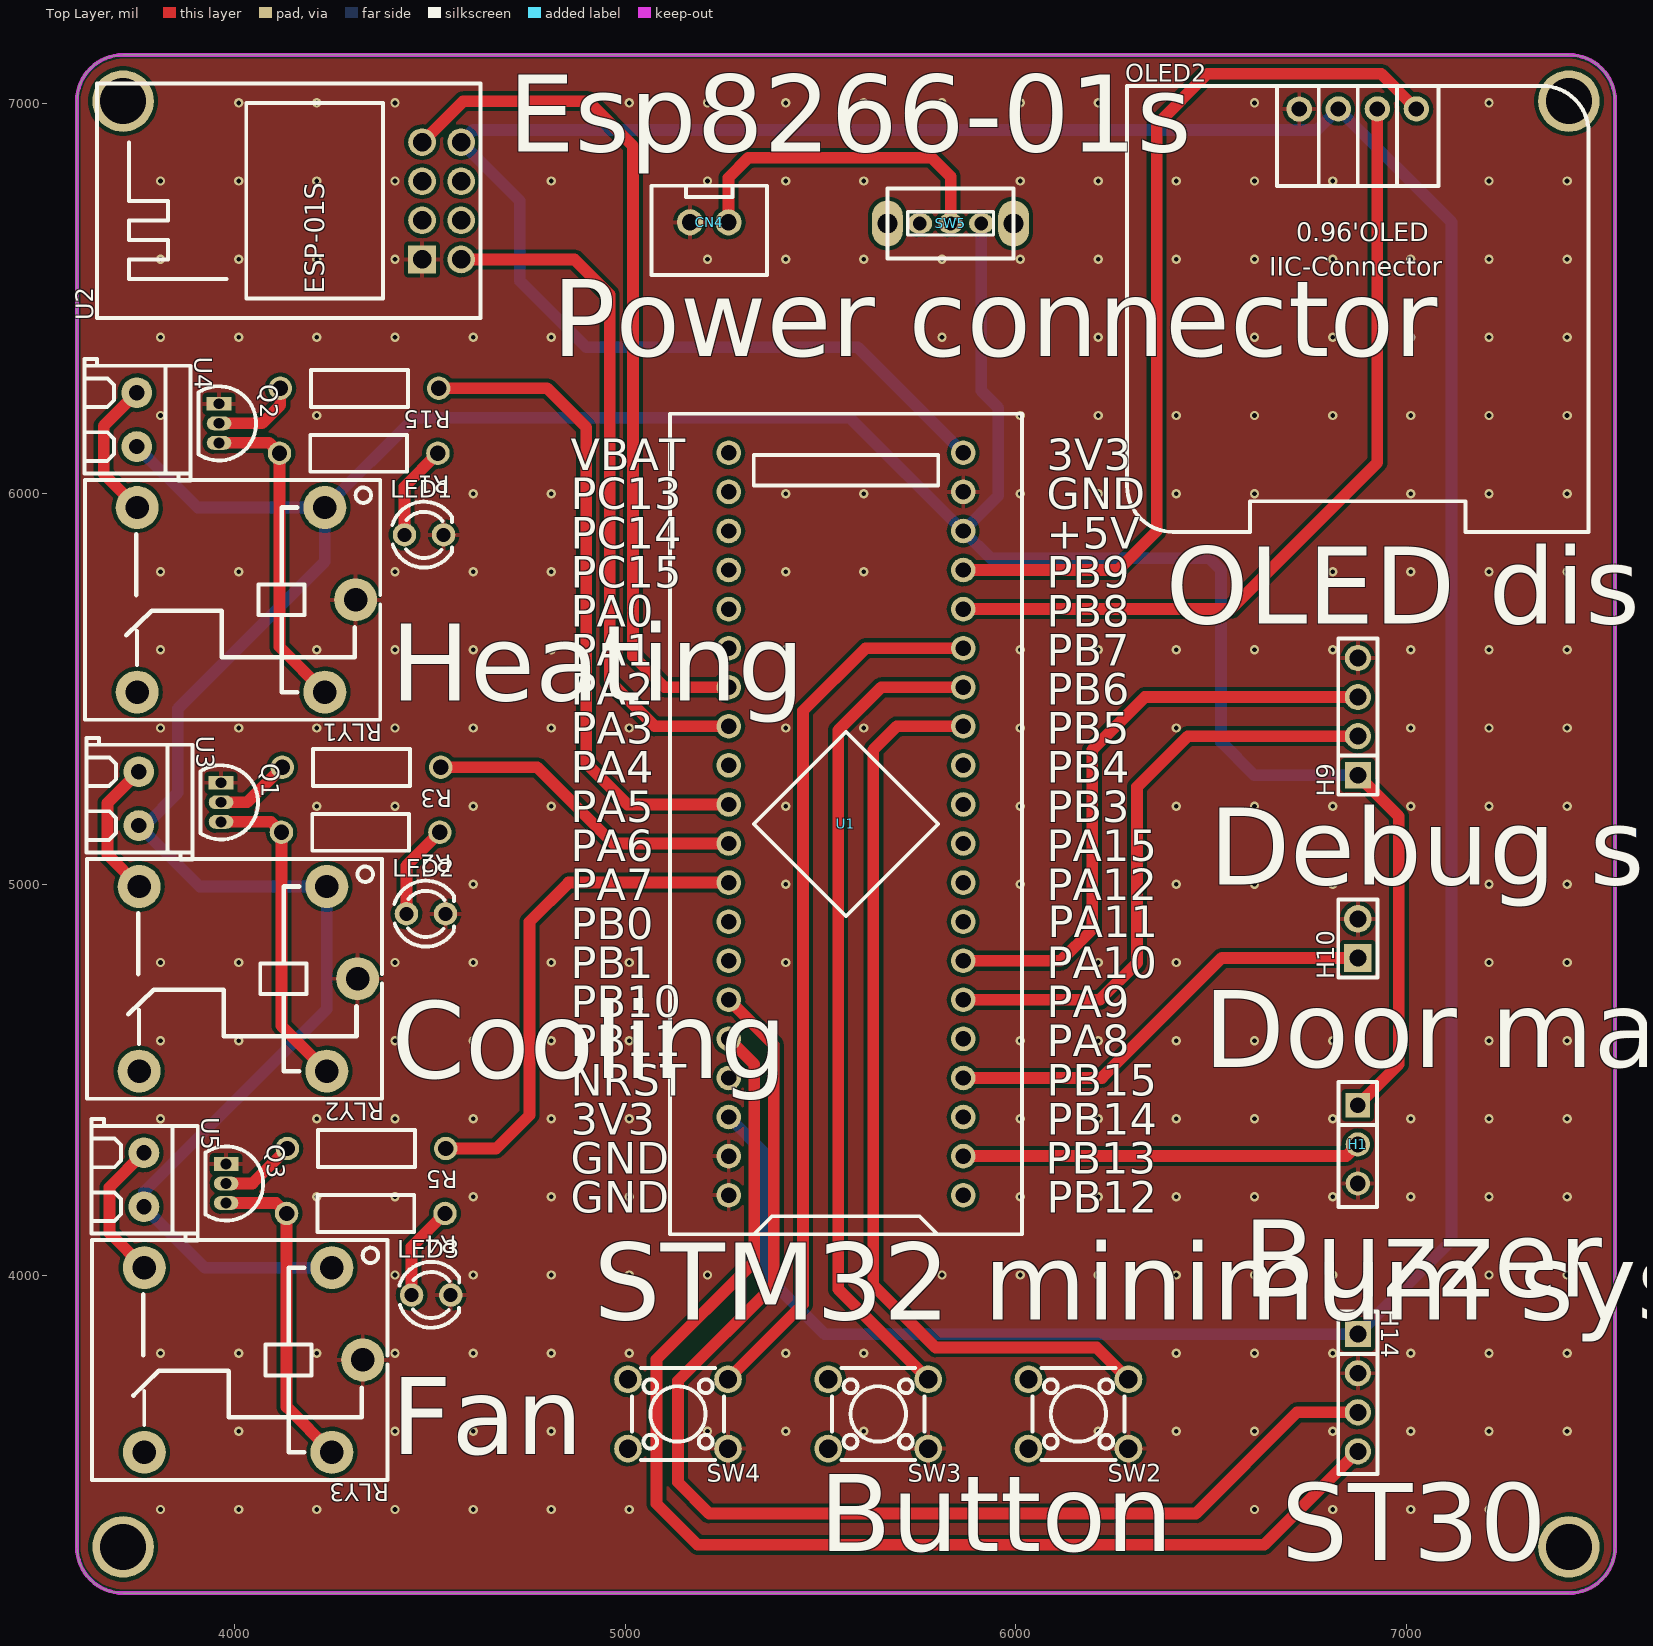
[diagram p0: Top Layer view]
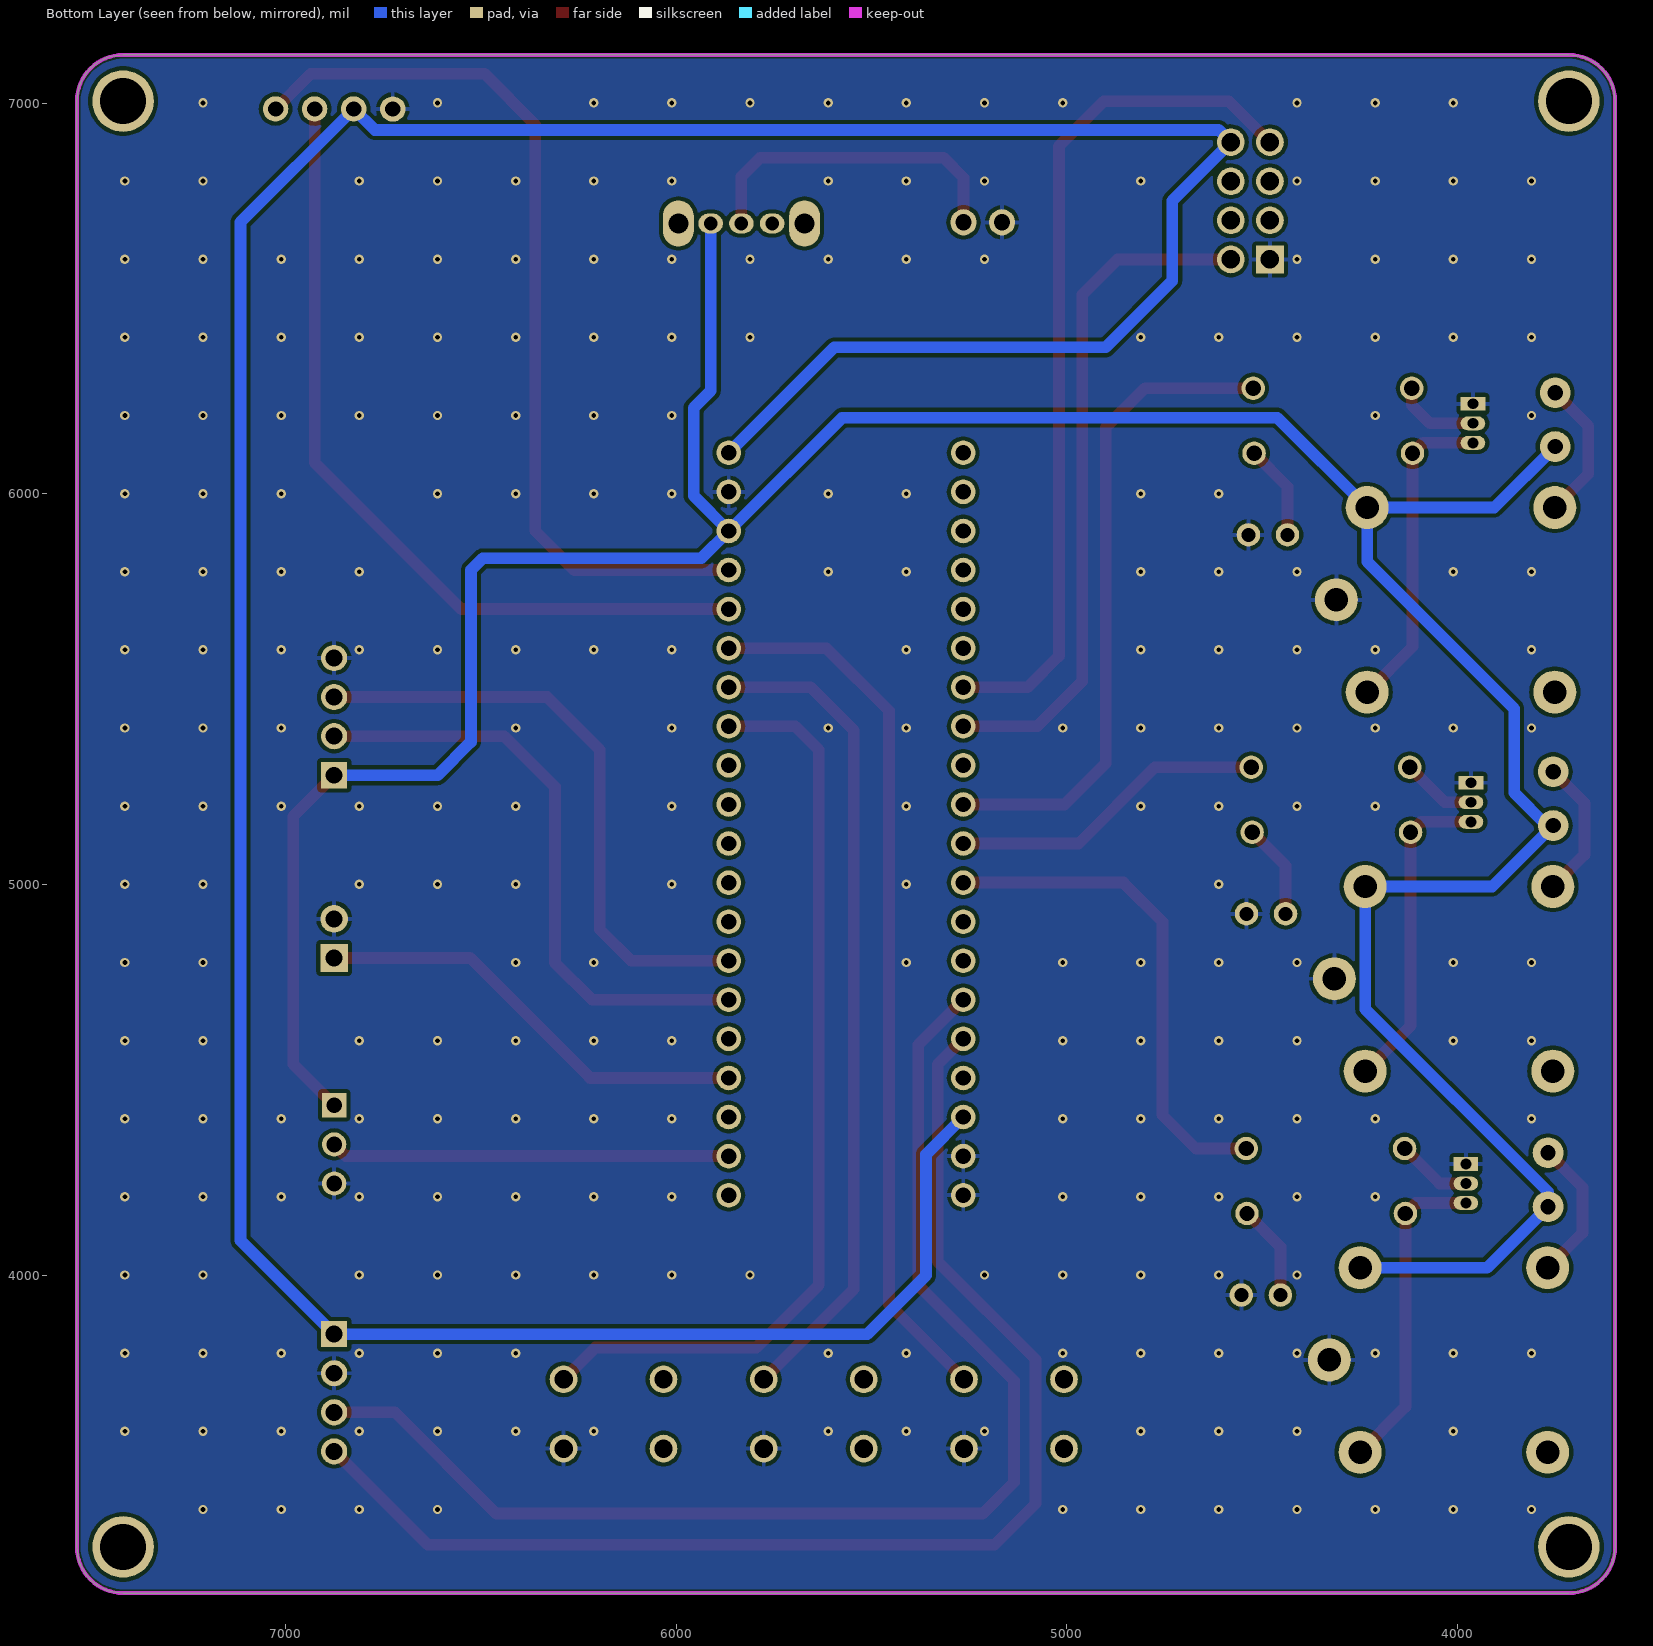
[diagram p1: Bottom Layer view, seen from below]
# Altium PCB MISC51783.pcbdoc
Units mil, origin at the board's own origin, x right, y up, seen from the top; angles counter-clockwise.
Board outline 3937.01 x 3937.01 mil, 2 copper layers (Top Layer, Bottom Layer), stack 62.206 mil thick; 30 components, 50 nets, 136 pads, 242 vias.

## Layer stack, top to bottom
Top Solder Mask Layer: solder mask 0.394, Dk 3.3
Top Layer: signal copper 1.379
Dielectric1: surface 59.449, FR4, Dk 4.5
Bottom Layer: signal copper 1.378
Bottom Solder Mask Layer: solder mask 0.394, Dk 3.3

## Board outline
3714.61,7123.5 ccw(c3714.61,7005.39) 3596.5,7005.39 3596.5,3304.61 ccw(c3714.61,3304.61) 3714.61,3186.5 7415.39,3186.5 ccw(c7415.39,3304.61) 7533.5,3304.61 7533.5,7005.39 ccw(c7415.39,7005.39) 7415.39,7123.5 3714.61,7123.5

## Design rules (kind name [scope] priority, off if disabled: settings)
BoardOutlineClearance copperThickness2oz_1 [All] p2 off: genericclearance=7.99 ignorepadtopadclearanceinfootprint=FALSE except(0: Arc-SplitContinuation Track-SplitContinuation SMDPad-SplitContinuation THPad-SplitContinuation Via-SplitContinuation Fill-SplitContinuation Region-SplitContinuation Poly-SplitContinuation Text-SplitContinuation Hole-SplitContinuation; 5.98: Arc-CutoutEdge Track-CutoutEdge SMDPad-CutoutEdge THPad-CutoutEdge Via-CutoutEdge Text-CutoutEdge; 6.9: Hole-OutlineEdge Hole-CutoutEdge; 10: Poly-OutlineEdge Poly-CutoutEdge; 11.81: Arc-OutlineEdge Track-OutlineEdge SMDPad-OutlineEdge THPad-OutlineEdge Via-OutlineEdge Fill-OutlineEdge Region-OutlineEdge Text-OutlineEdge Fill-CutoutEdge Region-CutoutEdge)
BoardOutlineClearance Plane_innerPlane_1 [All] p4 off: genericclearance=4.02 ignorepadtopadclearanceinfootprint=FALSE except(0: Arc-SplitContinuation Track-SplitContinuation SMDPad-SplitContinuation THPad-SplitContinuation Via-SplitContinuation Fill-SplitContinuation Region-SplitContinuation Poly-SplitContinuation Text-SplitContinuation Hole-SplitContinuation; 5.98: Arc-CutoutEdge Track-CutoutEdge SMDPad-CutoutEdge THPad-CutoutEdge Via-CutoutEdge Text-CutoutEdge; 6.9: Hole-OutlineEdge Hole-CutoutEdge; 10: Poly-OutlineEdge Poly-CutoutEdge; 11.81: Arc-OutlineEdge Track-OutlineEdge SMDPad-OutlineEdge THPad-OutlineEdge Via-OutlineEdge Fill-OutlineEdge Region-OutlineEdge Text-OutlineEdge Fill-CutoutEdge Region-CutoutEdge)
BoardOutlineClearance Copper_copperRegion_1 [All] p6 off: genericclearance=4.02 ignorepadtopadclearanceinfootprint=FALSE except(0: Arc-SplitContinuation Track-SplitContinuation SMDPad-SplitContinuation THPad-SplitContinuation Via-SplitContinuation Fill-SplitContinuation Region-SplitContinuation Poly-SplitContinuation Text-SplitContinuation Hole-SplitContinuation; 5.98: Arc-CutoutEdge Track-CutoutEdge SMDPad-CutoutEdge THPad-CutoutEdge Via-CutoutEdge Text-CutoutEdge; 6.9: Hole-OutlineEdge Hole-CutoutEdge; 10: Poly-OutlineEdge Poly-CutoutEdge; 11.81: Arc-OutlineEdge Track-OutlineEdge SMDPad-OutlineEdge THPad-OutlineEdge Via-OutlineEdge Fill-OutlineEdge Region-OutlineEdge Text-OutlineEdge Fill-CutoutEdge Region-CutoutEdge)
BoardOutlineClearance Copper_copperRegion_copperThickness1oz_1 [All] p8 off: genericclearance=4.02 ignorepadtopadclearanceinfootprint=FALSE except(0: Arc-SplitContinuation Track-SplitContinuation SMDPad-SplitContinuation THPad-SplitContinuation Via-SplitContinuation Fill-SplitContinuation Region-SplitContinuation Poly-SplitContinuation Text-SplitContinuation Hole-SplitContinuation; 5.98: Arc-CutoutEdge Track-CutoutEdge SMDPad-CutoutEdge THPad-CutoutEdge Via-CutoutEdge Text-CutoutEdge; 6.9: Hole-OutlineEdge Hole-CutoutEdge; 10: Poly-OutlineEdge Poly-CutoutEdge; 11.81: Arc-OutlineEdge Track-OutlineEdge SMDPad-OutlineEdge THPad-OutlineEdge Via-OutlineEdge Fill-OutlineEdge Region-OutlineEdge Text-OutlineEdge Fill-CutoutEdge Region-CutoutEdge)
BoardOutlineClearance Copper_copperRegion_Copper_copperRegion_1 [All] p10 off: genericclearance=4.02 ignorepadtopadclearanceinfootprint=FALSE except(0: Arc-SplitContinuation Track-SplitContinuation SMDPad-SplitContinuation THPad-SplitContinuation Via-SplitContinuation Fill-SplitContinuation Region-SplitContinuation Poly-SplitContinuation Text-SplitContinuation Hole-SplitContinuation; 5.98: Arc-CutoutEdge Track-CutoutEdge SMDPad-CutoutEdge THPad-CutoutEdge Via-CutoutEdge Text-CutoutEdge; 6.9: Hole-OutlineEdge Hole-CutoutEdge; 10: Poly-OutlineEdge Poly-CutoutEdge; 11.81: Arc-OutlineEdge Track-OutlineEdge SMDPad-OutlineEdge THPad-OutlineEdge Via-OutlineEdge Fill-OutlineEdge Region-OutlineEdge Text-OutlineEdge Fill-CutoutEdge Region-CutoutEdge)
BoardOutlineClearance copperThickness1oz_1 [All] p12: genericclearance=4.02 ignorepadtopadclearanceinfootprint=FALSE except(0: Arc-SplitContinuation Track-SplitContinuation SMDPad-SplitContinuation THPad-SplitContinuation Via-SplitContinuation Fill-SplitContinuation Region-SplitContinuation Poly-SplitContinuation Text-SplitContinuation Hole-SplitContinuation; 5.98: Arc-CutoutEdge Track-CutoutEdge SMDPad-CutoutEdge THPad-CutoutEdge Via-CutoutEdge Text-CutoutEdge; 6.9: Hole-OutlineEdge Hole-CutoutEdge; 10: Poly-OutlineEdge Poly-CutoutEdge; 11.81: Arc-OutlineEdge Track-OutlineEdge SMDPad-OutlineEdge THPad-OutlineEdge Via-OutlineEdge Fill-OutlineEdge Region-OutlineEdge Text-OutlineEdge Fill-CutoutEdge Region-CutoutEdge)
Clearance copperThickness2oz [All] p1 off: gap=7.99 ignorepadtopadclearanceinfootprint=FALSE except(5.98: SMDPad-Track SMDPad-SMDPad THPad-Track SMDPad-THPad THPad-THPad Track-Via SMDPad-Via THPad-Via Via-Via Fill-SMDPad Region-SMDPad Fill-THPad Region-THPad Fill-Via Region-Via Fill-Fill Fill-Region Region-Region Arc-Track Arc-SMDPad Arc-THPad Arc-Via Fill-Arc Region-Arc Arc-Arc Text-Track SMDPad-Text Text-THPad Text-Via Fill-Text Region-Text Arc-Text Text-Text; 6.9: Hole-Track Hole-SMDPad Hole-THPad Hole-Via Fill-Hole Region-Hole Hole-Arc Hole-Text; 10: Poly-Track Poly-SMDPad Poly-THPad Poly-Via Poly-Fill Poly-Region Poly-Poly Poly-Arc Poly-Text Poly-Hole; 11.81: Fill-Track Region-Track)
Clearance Plane_innerPlane [All] p3 off: gap=4.02 ignorepadtopadclearanceinfootprint=FALSE except(5.98: SMDPad-Track SMDPad-SMDPad THPad-Track SMDPad-THPad THPad-THPad Track-Via SMDPad-Via THPad-Via Via-Via Fill-SMDPad Region-SMDPad Fill-THPad Region-THPad Fill-Via Region-Via Fill-Fill Fill-Region Region-Region Arc-Track Arc-SMDPad Arc-THPad Arc-Via Fill-Arc Region-Arc Arc-Arc Text-Track SMDPad-Text Text-THPad Text-Via Fill-Text Region-Text Arc-Text Text-Text; 6.9: Hole-Track Hole-SMDPad Hole-THPad Hole-Via Fill-Hole Region-Hole Hole-Arc Hole-Text; 10: Poly-Track Poly-SMDPad Poly-THPad Poly-Via Poly-Fill Poly-Region Poly-Poly Poly-Arc Poly-Text Poly-Hole; 11.81: Fill-Track Region-Track)
Clearance Copper_copperRegion [All] p5 off: gap=4.02 ignorepadtopadclearanceinfootprint=FALSE except(5.98: SMDPad-Track SMDPad-SMDPad THPad-Track SMDPad-THPad THPad-THPad Track-Via SMDPad-Via THPad-Via Via-Via Fill-SMDPad Region-SMDPad Fill-THPad Region-THPad Fill-Via Region-Via Fill-Fill Fill-Region Region-Region Arc-Track Arc-SMDPad Arc-THPad Arc-Via Fill-Arc Region-Arc Arc-Arc Text-Track SMDPad-Text Text-THPad Text-Via Fill-Text Region-Text Arc-Text Text-Text; 6.9: Hole-Track Hole-SMDPad Hole-THPad Hole-Via Fill-Hole Region-Hole Hole-Arc Hole-Text; 10: Poly-Track Poly-SMDPad Poly-THPad Poly-Via Poly-Fill Poly-Region Poly-Poly Poly-Arc Poly-Text Poly-Hole; 11.81: Fill-Track Region-Track)
Clearance Copper_copperRegion_copperThickness1oz [All] p7 off: gap=4.02 ignorepadtopadclearanceinfootprint=FALSE except(5.98: SMDPad-Track SMDPad-SMDPad THPad-Track SMDPad-THPad THPad-THPad Track-Via SMDPad-Via THPad-Via Via-Via Fill-SMDPad Region-SMDPad Fill-THPad Region-THPad Fill-Via Region-Via Fill-Fill Fill-Region Region-Region Arc-Track Arc-SMDPad Arc-THPad Arc-Via Fill-Arc Region-Arc Arc-Arc Text-Track SMDPad-Text Text-THPad Text-Via Fill-Text Region-Text Arc-Text Text-Text; 6.9: Hole-Track Hole-SMDPad Hole-THPad Hole-Via Fill-Hole Region-Hole Hole-Arc Hole-Text; 10: Poly-Track Poly-SMDPad Poly-THPad Poly-Via Poly-Fill Poly-Region Poly-Poly Poly-Arc Poly-Text Poly-Hole; 11.81: Fill-Track Region-Track)
Clearance Copper_copperRegion_Copper_copperRegion [All] p9 off: gap=4.02 ignorepadtopadclearanceinfootprint=FALSE except(5.98: SMDPad-Track SMDPad-SMDPad THPad-Track SMDPad-THPad THPad-THPad Track-Via SMDPad-Via THPad-Via Via-Via Fill-SMDPad Region-SMDPad Fill-THPad Region-THPad Fill-Via Region-Via Fill-Fill Fill-Region Region-Region Arc-Track Arc-SMDPad Arc-THPad Arc-Via Fill-Arc Region-Arc Arc-Arc Text-Track SMDPad-Text Text-THPad Text-Via Fill-Text Region-Text Arc-Text Text-Text; 6.9: Hole-Track Hole-SMDPad Hole-THPad Hole-Via Fill-Hole Region-Hole Hole-Arc Hole-Text; 10: Poly-Track Poly-SMDPad Poly-THPad Poly-Via Poly-Fill Poly-Region Poly-Poly Poly-Arc Poly-Text Poly-Hole; 11.81: Fill-Track Region-Track)
Clearance copperThickness1oz [All] p11: gap=4.02 ignorepadtopadclearanceinfootprint=FALSE except(5.98: SMDPad-Track SMDPad-SMDPad THPad-Track SMDPad-THPad THPad-THPad Track-Via SMDPad-Via THPad-Via Via-Via Fill-SMDPad Region-SMDPad Fill-THPad Region-THPad Fill-Via Region-Via Fill-Fill Fill-Region Region-Region Arc-Track Arc-SMDPad Arc-THPad Arc-Via Fill-Arc Region-Arc Arc-Arc Text-Track SMDPad-Text Text-THPad Text-Via Fill-Text Region-Text Arc-Text Text-Text; 6.9: Hole-Track Hole-SMDPad Hole-THPad Hole-Via Fill-Hole Region-Hole Hole-Arc Hole-Text; 10: Poly-Track Poly-SMDPad Poly-THPad Poly-Via Poly-Fill Poly-Region Poly-Poly Poly-Arc Poly-Text Poly-Hole; 11.81: Fill-Track Region-Track)
DiffPairsRouting differentialPair [All] p1: maxlimit=6 minlimit=6 mostfreqgap=6 toplayer_minwidth=5 toplayer_prefwidth=10 toplayer_maxwidth=100 toplayer_mingap=6 toplayer_prefgap=6 toplayer_maxgap=6 bottomlayer_minwidth=5 bottomlayer_prefwidth=10 bottomlayer_maxwidth=100 bottomlayer_mingap=6 bottomlayer_prefgap=6 bottomlayer_maxgap=6 maxuncoupledlength=10
HoleToHoleClearance otherClearance [All] p1: gap=11.81 allowstackedmicrovias=TRUE
Length netLength [All] p1: minlimit=0 maxlimit=0
PasteMaskExpansion pasteMaskExpansion [All] p1: expansion=0
PlaneConnect innerPlane [All] p1: planeconnectstyle=Relief reliefexpansion=20 reliefentries=4 reliefconductorwidth=10 reliefairgap=10
PolygonConnect copperRegion_copperThickness1oz [All] p1 off: connectstyle=Relief reliefconductorwidth=10 reliefentries=4 polygonreliefangle="90 Angle" airgapwidth=10 via.connectstyle=Relief via.reliefconductorwidth=10 via.reliefentries=4 via.polygonreliefangle="90 Angle" via.airgapwidth=10
PolygonConnect copperRegion_Copper_copperRegion [All] p2 off: connectstyle=Relief reliefconductorwidth=10 reliefentries=4 polygonreliefangle="90 Angle" airgapwidth=10 via.connectstyle=Relief via.reliefconductorwidth=10 via.reliefentries=4 via.polygonreliefangle="90 Angle" via.airgapwidth=10
PolygonConnect copperRegion [All] p3: connectstyle=Relief reliefconductorwidth=10 reliefentries=4 polygonreliefangle="90 Angle" airgapwidth=10 via.connectstyle=Relief via.reliefconductorwidth=10 via.reliefentries=4 via.polygonreliefangle="90 Angle" via.airgapwidth=10
RoutingVias viaSize [All] p1: holewidth=12.01 width=24.02 viastyle="Through Hole" minholewidth=11.81 minwidth=19.68 maxholewidth=248.03 maxwidth=393.7
SolderMaskExpansion solderMaskExpansion [IsVia] p1: expansion=-1000 istentingtop=TRUE
SolderMaskExpansion solderMaskExpansion [All] p2: expansion=2 istentingtop=FALSE
Width copperThickness2oz_2 [All] p1 off: maxlimit=100 minlimit=8 preferedwidth=10
Width copperThickness1oz_2 [All] p2: maxlimit=100 minlimit=5 preferedwidth=10

## Components (designator, comment, footprint, x,y, rotation, side; value= is the part's Value field where it differs from the comment)
CN4 "XH2.54*2P_THT" CONN-TH_2P-P2.50-XH2.54-2P 5215,6695 r0 top
H1 "" HDR-TH_3P-P2.54-V-F 6875,4334.89 r270 top
H9 "" HDR-TH_4P-P2.54-V-M 6875,5429.77 r90 top
H10 "" HDR-TH_2P-P2.54-V-M-1 6875,4862.25 r90 top
H14 "" HDR-TH_4P-P2.54-V-F 6875,3699.27 r270 top
LED1 "" LED_TH-3mm 4485,5895 r0 top
LED2 "" LED_TH-3mm 4490,4925 r0 top
LED3 "" LED_TH-3mm 4503.13,3949.41 r0 top
OLED2 "" 0.96OLED_4P 6875,6985 r0 top
Q1 "" S8050_TO_92 3965.37,5210.48 r270 top
Q2 "" S8050_TO_92 3960.37,6180.48 r270 top
Q3 "" S8050_TO_92 3978.5,4234.89 r270 top
R1 "1kΩ" Res_1/4W 4317.81,6103.81 r180 top
R2 "1kΩ" Res_1/4W 4322.81,5133.81 r180 top
R3 "1kΩ" Res_1/4W 4325,5300 r180 top
R4 "1kΩ" Res_1/4W 4335.94,4158.22 r180 top
R5 "1kΩ" Res_1/4W 4338.13,4324.41 r180 top
R15 "1kΩ" Res_1/4W 4320,6270 r180 top
RLY1 "SRD-05VDC-SL-C" RELAY-TH_SRD-XXVDC-XL-C 4030.37,5728.81 r180 top
RLY2 "SRD-05VDC-SL-C" RELAY-TH_SRD-XXVDC-XL-C 4035.37,4758.81 r180 top
RLY3 "SRD-05VDC-SL-C" RELAY-TH_SRD-XXVDC-XL-C 4048.5,3783.22 r180 top
SW2 "" SW-TH_4P-L6.0-W6.0-P4.50-LS6.5 6160,3645 r180 top
SW3 "" SW-TH_4P-L6.0-W6.0-P4.50-LS6.5 5647.5,3645 r180 top
SW4 "" SW-TH_4P-L6.0-W6.0-P4.50-LS6.5 5135,3645 r180 top
SW5 "" 拨动开关 5837.9,6692.05 r180 top
U1 "STM32F103C8T6-Card" CONN-TH_L53.3-W22.9_STM32F103C8T6-CARD 5565,5155 r90 top
U2 "ESP-01S" WIFIM-TH_ESP-01S 4530,6750 r90 top
U3 "KF350-3.5-2P" CONN-TH_P3.50_KF350-3.5-2P 3755,5220 r270 top
U4 "KF350-3.5-2P" CONN-TH_P3.50_KF350-3.5-2P 3750,6190 r270 top
U5 "KF350-3.5-2P" CONN-TH_P3.50_KF350-3.5-2P 3768.13,4244.41 r270 top

## Footprints (in the part's own frame and the unit in brackets; to place one, negate y for a bottom-side part, rotate by r counter-clockwise, add the part's x,y. Pads: shape width x height; smd on the part's side, far side on the other; paste and mask are expansions set on the pad)
0.96OLED_4P [mm]
  round 1.65 hole 1 copper offset 0,0: 1(-3.81,-0.001) 2(-1.27,0.002) 3(1.27,0.002) 4(3.81,0.002)
  silkscreen extent -15,-27.5 15,1.5
CONN-TH_2P-P2.50-XH2.54-2P [mm]
  round 1.7 hole 1.05 paste+0 mask+0.05: 1(1.25,0) 2(-1.25,0)
  silkscreen extent -3.75,-3.42 3.75,2.37
CONN-TH_L53.3-W22.9_STM32F103C8T6-CARD [mm]
  round 1.6 hole 1: 1(-24.13,-7.62) 2(-21.59,-7.62) 3(-19.05,-7.62) 4(-16.51,-7.62) 5(-13.97,-7.62) 6(-11.43,-7.62) 7(-8.89,-7.62) 8(-6.35,-7.62) 9(-3.81,-7.62) 10(-1.27,-7.62) 11(1.27,-7.62) 12(3.81,-7.62) 13(6.35,-7.62) 14(8.89,-7.62) 15(11.43,-7.62) 16(13.97,-7.62) 17(16.51,-7.62) 18(19.05,-7.62) 19(21.59,-7.62) 20(24.13,-7.62) 21(24.13,7.62) 22(21.59,7.62) 23(19.05,7.62) 24(16.51,7.62) 25(13.97,7.62) 26(11.43,7.62) 27(8.89,7.62) 28(6.35,7.62) 29(3.81,7.62) 30(1.27,7.62) 31(-1.27,7.62) 32(-3.81,7.62) 33(-6.35,7.62) 34(-8.89,7.62) 35(-11.43,7.62) 36(-13.97,7.62) 37(-16.51,7.62) 38(-19.05,7.62) 39(-21.59,7.62) 40(-24.13,7.62)
  silkscreen extent -26.67,-11.43 26.67,11.43
CONN-TH_P3.50_KF350-3.5-2P [mm]
  round 2 hole 1: 1(-1.75,0) 2(1.75,0)
  silkscreen extent -3.95,-3.4 3.95,3.5
HDR-TH_2P-P2.54-V-M-1 [mm]
  rect 1.8x1.8 hole 1.1: 1(-1.27,0)
  round 1.8 hole 1.1: 2(1.27,0)
  silkscreen extent -2.54,-1.27 2.54,1.27
HDR-TH_3P-P2.54-V-F [mil]
  rect 62x62 hole 40.16: 1(-100,0)
  round 62 hole 40.16: 2(0,0) 3(100,0)
  silkscreen extent -160,-49 160,49
HDR-TH_4P-P2.54-V-F [mm]
  rect 1.7x1.7 hole 1.1: 1(-3.81,0)
  round 1.7 hole 1.1: 2(-1.27,0) 3(1.27,0) 4(3.81,0)
  silkscreen extent -5.29,-1.27 5.29,1.27
HDR-TH_4P-P2.54-V-M [mm]
  rect 1.7x1.7 hole 1.1: 1(-3.81,0)
  round 1.7 hole 1.1: 2(-1.27,0) 3(1.27,0) 4(3.81,0)
  silkscreen extent -5.08,-1.27 5.08,1.27
LED_TH-3mm [mil]
  round 60 hole 36 paste+0 mask+2: 1(-50,0) 2(50,0)
  silkscreen extent -81,-84 72,85
RELAY-TH_SRD-XXVDC-XL-C [mil]
  round 110 hole 60: 1(-200.79,-236.22) 2(279.53,-236.2) 3(279.53,236.2) 4(-200.79,236.22) 5(-279.53,0)
  silkscreen extent -342,-307 413,307
Res_1/4W [mil]
  round 60 hole 39.37 paste+0 mask+2: 1(-202.76,0) 2(202.76,0)
  silkscreen extent -124,-47 124,47
S8050_TO_92 [mil]
  rect 35.4x63 hole 27.6 paste+0 mask+2: 1(-50,0)
  oval 35.4x63 hole 27.6 paste+0 mask+2: 2(0,0) 3(50,0)
  silkscreen extent -95,-53 95,95
SW-TH_4P-L6.0-W6.0-P4.50-LS6.5 [mm]
  round 1.8 hole 1.2: 1(-3.25,2.25) 2(3.25,2.25) 3(-3.25,-2.25) 4(3.25,-2.25)
  silkscreen extent -3,-3 3,3
WIFIM-TH_ESP-01S [mm]
  rect 1.8x1.8 hole 1.2: 1(-3.81,1.27)
  round 1.8 hole 1.2: 2(-1.27,1.27) 3(1.27,1.27) 4(3.81,1.27) 5(3.81,-1.27) 6(1.27,-1.27) 7(-1.27,-1.27) 8(-3.81,-1.27)
  silkscreen extent -7.62,-2.54 7.62,22.4
拨动开关 [mil]
  oval 63x51.2 hole 35.4 paste+0 mask+2: 1(-73.4,0) 2(5,0) 3(84,0)
  oval 78.7x118.1 hole 51.2 paste+0 mask+2: 4(166.7,0) 5(-156.1,0)
  silkscreen extent -156,-90 167,90

## Free pads (board coordinates)
  round 157.48 hole 118.11: 1(3714.61,7005.39) 1(3714.61,3304.61) 1(7415.39,7005.39) 1(7415.39,3304.61)

## Via types
v1: diameter 24.02, hole 12, Top Layer to Bottom Layer, 242 vias

## Nets (pads, with @x,y where several pads share a name; then routed paths per layer and width w, separated by ;. In a path a pad name is that pad's centre, name@x,y a point inside that pad or via, vN(x,y) a via of type N, cw(c..) or ccw(c..) an arc to the next point about the centre after c; other vN are vias at no path point)
$1N17118: CN4.1 SW5.2 | length 843.8
  Top Layer w30: CN4.1 5264.22,6809.22 5315,6860 5785,6860 5832.9,6812.1 SW5.2
$1N17196: Q2.2 R15.2 | length 219
  Top Layer w30: Q2.2 4070.48,6180.48 4117.24,6227.24 R15.2
$1N17201: RLY1.2 U4.1 | length 364.6
  Top Layer w30: U4.1 3665,6173.9 3665,6050.85 RLY1.2
$1N17203: LED1.1 R1.1 | length 244.3
  Top Layer w30: LED1.1 4435,6018.24 R1.1
$1N17204: Q2.3 R1.2 RLY1.4 | length 825
  Top Layer w30: Q2.3 4088.38,6130.48 R1.2 4115.05,5608.7 RLY1.4
$1N17207: Q1.3 R2.2 RLY2.4 | length 825
  Top Layer w30: Q1.3 4093.38,5160.48 R2.2 4120.05,4638.7 RLY2.4
$1N17208: LED2.1 R2.1 | length 244.3
  Top Layer w30: LED2.1 4440,5048.24 R2.1
$1N17210: Q1.2 R3.2 | length 194
  Top Layer w30: Q1.2 4032.72,5210.48 R3.2
$1N17214: RLY2.2 U3.1 | length 360.5
  Top Layer w30: U3.1 3675,5208.9 3675,5075.85 RLY2.2
$1N17217: Q3.3 R4.2 RLY3.4 | length 825
  Top Layer w30: Q3.3 4106.52,4184.89 R4.2 4133.19,3663.1 RLY3.4
$1N17218: LED3.1 R4.1 | length 244.3
  Top Layer w30: LED3.1 4453.13,4072.64 R4.1
$1N17220: Q3.2 R5.2 | length 194
  Top Layer w30: Q3.2 4045.85,4234.89 R5.2
$1N17224: RLY3.2 U5.1 | length 367.2
  Top Layer w30: U5.1 3680,4225.17 3680,4108.39 RLY3.2
+5V: H1.1 H9.1 RLY1.1 RLY2.1 RLY3.1 SW5.1 U1.18 U3.2 U4.2 U5.2 | length 8821.6
  Top Layer w30: H1.1 6980,4539.9 6980,5174.76 H9.1
  Bottom Layer w30: U4.2 3906.08,5965.03 RLY1.1 ; RLY3.1 3924.21,4019.44 U5.2 3768.13,4213.13 4236.16,4681.16 RLY2.1 3911.08,4995.03 U3.2 3771.11,5151.11 3855,5235 3855,5450 4231.16,5826.16 RLY1.1 ; SW5.1 5911.3,6263.7 5955,6220 5955,5995 U1.18 ; H9.1 6610.23,5279.77 6525,5365 6525,5805 6495,5835 5935,5835 U1.18 ; RLY1.1 4461.13,6195 5575,6195 U1.18
GND: CN4.2 H1.3 H9.4 H10.2 H14.2 LED1.2 LED2.2 LED3.2 OLED2.1 Q1.1 Q2.1 Q3.1 RLY1.5 RLY2.5 RLY3.5 SW2.1 SW3.1 SW4.1 U1.19 U1.39 U1.40 U2.1
  other v1: 3810.6,3400.6 4010.6,3400.6 4210.6,3400.6 4410.6,3400.6 4610.6,3400.6 4810.6,3400.6 5010.6,3400.6 6610.6,3400.6 6810.6,3400.6 7010.6,3400.6 7210.6,3400.6 4010.6,3600.6 4410.6,3600.6 4610.6,3600.6 4810.6,3600.6 5210.6,3600.6 5410.6,3600.6 5610.6,3600.6 6210.6,3600.6 6410.6,3600.6 6610.6,3600.6 6810.6,3600.6 7010.6,3600.6 7210.6,3600.6 7410.6,3600.6 3810.6,3800.6 4010.6,3800.6 4210.6,3800.6 4410.6,3800.6 4610.6,3800.6 4810.6,3800.6 5010.6,3800.6 5410.6,3800.6 5610.6,3800.6 6410.6,3800.6 6610.6,3800.6 6810.6,3800.6 7010.6,3800.6 7210.6,3800.6 7410.6,3800.6 4410.6,4000.6 4610.6,4000.6 4810.6,4000.6 5010.6,4000.6 5210.6,4000.6 5810.6,4000.6 6010.6,4000.6 6210.6,4000.6 6410.6,4000.6 6610.6,4000.6 6810.6,4000.6 7210.6,4000.6 7410.6,4000.6 4210.6,4200.6 4410.6,4200.6 4610.6,4200.6 4810.6,4200.6 5010.6,4200.6 6010.6,4200.6 6210.6,4200.6 6410.6,4200.6 6610.6,4200.6 6810.6,4200.6 7010.6,4200.6 7210.6,4200.6 7410.6,4200.6 3810.6,4400.6 4210.6,4400.6 4410.6,4400.6 4610.6,4400.6 4810.6,4400.6 5010.6,4400.6 6010.6,4400.6 6210.6,4400.6 6410.6,4400.6 6610.6,4400.6 6810.6,4400.6 7010.6,4400.6 7210.6,4400.6 7410.6,4400.6 3810.6,4600.6 4010.6,4600.6 4410.6,4600.6 4610.6,4600.6 4810.6,4600.6 5010.6,4600.6 6010.6,4600.6 6210.6,4600.6 6410.6,4600.6 6610.6,4600.6 6810.6,4600.6 7210.6,4600.6 7410.6,4600.6 3810.6,4800.6 4010.6,4800.6 4410.6,4800.6 4610.6,4800.6 4810.6,4800.6 5010.6,4800.6 5410.6,4800.6 6210.6,4800.6 6410.6,4800.6 7210.6,4800.6 7410.6,4800.6 4610.6,5000.6 5410.6,5000.6 6010.6,5000.6 6410.6,5000.6 6610.6,5000.6 6810.6,5000.6 7210.6,5000.6 7410.6,5000.6 4210.6,5200.6 4410.6,5200.6 4610.6,5200.6 4810.6,5200.6 5410.6,5200.6 6010.6,5200.6 6410.6,5200.6 6610.6,5200.6 6810.6,5200.6 7010.6,5200.6 7210.6,5200.6 7410.6,5200.6 3810.6,5400.6 4010.6,5400.6 4210.6,5400.6 4410.6,5400.6 4610.6,5400.6 4810.6,5400.6 5010.6,5400.6 5410.6,5400.6 5610.6,5400.6 6010.6,5400.6 6410.6,5400.6 7010.6,5400.6 7210.6,5400.6 7410.6,5400.6 3810.6,5600.6 4210.6,5600.6 4410.6,5600.6 4610.6,5600.6 4810.6,5600.6 5410.6,5600.6 6010.6,5600.6 6210.6,5600.6 6410.6,5600.6 6610.6,5600.6 6810.6,5600.6 7010.6,5600.6 7210.6,5600.6 7410.6,5600.6 3810.6,5800.6 4010.6,5800.6 4410.6,5800.6 4610.6,5800.6 4810.6,5800.6 5410.6,5800.6 5610.6,5800.6 6810.6,5800.6 7010.6,5800.6 7210.6,5800.6 7410.6,5800.6 4610.6,6000.6 4810.6,6000.6 5410.6,6000.6 5610.6,6000.6 6010.6,6000.6 6210.6,6000.6 6410.6,6000.6 6610.6,6000.6 7010.6,6000.6 7210.6,6000.6 7410.6,6000.6 3810.6,6200.6 4210.6,6200.6 6010.6,6200.6 6210.6,6200.6 6410.6,6200.6 6610.6,6200.6 6810.6,6200.6 7010.6,6200.6 7210.6,6200.6 7410.6,6200.6 3810.6,6400.6 4010.6,6400.6 4210.6,6400.6 4410.6,6400.6 4610.6,6400.6 4810.6,6400.6 5810.6,6400.6 6010.6,6400.6 6210.6,6400.6 6410.6,6400.6 6610.6,6400.6 6810.6,6400.6 7010.6,6400.6 7210.6,6400.6 7410.6,6400.6 3810.6,6600.6 4010.6,6600.6 4210.6,6600.6 4410.6,6600.6 5210.6,6600.6 5410.6,6600.6 5610.6,6600.6 5810.6,6600.6 6010.6,6600.6 6210.6,6600.6 6410.6,6600.6 6610.6,6600.6 6810.6,6600.6 7010.6,6600.6 7210.6,6600.6 7410.6,6600.6 3810.6,6800.6 4010.6,6800.6 4210.6,6800.6 4410.6,6800.6 4810.6,6800.6 5210.6,6800.6 5410.6,6800.6 5610.6,6800.6 6010.6,6800.6 6210.6,6800.6 6410.6,6800.6 6610.6,6800.6 6810.6,6800.6 7210.6,6800.6 7410.6,6800.6 4010.6,7000.6 4210.6,7000.6 4410.6,7000.6 5010.6,7000.6 5210.6,7000.6 5410.6,7000.6 5610.6,7000.6 5810.6,7000.6 6010.6,7000.6 6210.6,7000.6 6610.6,7000.6 7210.6,7000.6
NRST: U1.37
PA0: U1.25
PA1: U1.26
PA2: U1.27 U2.4 | length 2214.3
  Top Layer w30: U2.4 4585,7005 4905,7005 5020,6890 5020,5585 5100,5505 U1.27
PA3: U1.28 U2.8 | length 1759.9
  Top Layer w30: U2.8 4870,6600 4960,6510 4960,5520 5075,5405 U1.28
PA4: U1.29
PA5: R15.1 U1.30 | length 1687.2
  Top Layer w30: R15.1 4800,6270 4900,6170 4900,5310 5005,5205 U1.30
PA6: R3.1 U1.31 | length 818
  Top Layer w30: R3.1 4775,5300 4970,5105 U1.31
PA7: R5.1 U1.32 | length 1296
  Top Layer w30: R5.1 4669.41,4324.41 4755,4410 4755,4905 4855,5005 U1.32
PA8: U1.5
PA9: H9.2 U1.6 | length 1553.1
  Top Layer w30: U1.6 6215,4705 6310,4800 6310,5250 6439.77,5379.77 H9.2
PA10: H9.3 U1.7 | length 1559
  Top Layer w30: U1.7 6115,4805 6195,4885 6195,5345 6329.77,5479.77 H9.3
PA11: U1.8
PA12: U1.9
PA15: U1.10
PB0: U1.33
PB1: U1.34
PB3: U1.11
PB4: U1.12
PB5: SW2.3 U1.13 | length 2377.8
  Top Layer w30: U1.13 5695,5405 5635,5345 5635,3975 5795,3815 6206.53,3815 SW2.3
PB6: SW3.3 U1.14 | length 2122.4
  Top Layer w30: SW3.3@5775.45,3733.58 5545,3964.03 5545,5395 5655,5505 U1.14
PB7: SW4.3 U1.15 | length 2267.2
  Top Layer w30: SW4.3 5455,3925.63 5455,5445 5615,5605 U1.15
PB8: OLED2.3 U1.16 | length 2120.4
  Top Layer w30: U1.16 6550,5705 6925,6080 OLED2.3@6925,6985.05
PB9: OLED2.4 U1.17 | length 2332.5
  Top Layer w30: U1.17 6260,5805 6360,5905 6360,6945 6490,7075 6935.05,7075 OLED2.4@7025,6985.05
PB10: H14.3 U1.35 | length 3264.6
  Top Layer w30: U1.35 5380,4590 5380,3975 5135,3730 5135,3470 5215,3390 6460,3390 6719.27,3649.27 H14.3
PB11: H14.4 U1.36 | length 3258.1
  Top Layer w30: U1.36 5330,4540 5330,4035 5080,3785 5080,3415 5185,3310 6635.73,3310 H14.4
PB12: U1.1
PB13: H1.2 U1.2 | length 1022.4
  Top Layer w30: U1.2 6845.1,4305 H1.2
PB14: U1.3
PB15: H10.1 U1.4 | length 1137.3
  Top Layer w30: U1.4 6220,4505 6527.25,4812.25 H10.1
PC13: U1.22
PC14: U1.23
PC15: U1.24
VBAT: U1.21
VCC: H14.1 OLED2.2 U1.20 U1.38 U2.5 | length 9391.7
  Bottom Layer w30: U1.38 5360,4310 5360,4000 5510.73,3849.27 H14.1 7115,4089.27 7115,6695.05 6825,6985.05 6771.44,6931.49 4611.49,6931.49 U2.5 4730,6750 4730,6545 4900,6375 5595,6375 U1.20
pads on no net: RLY1.3 RLY2.3 RLY3.3 SW2.2 SW2.4 SW3.2 SW3.4 SW4.2 SW4.4 SW5.3 SW5.4 SW5.5 U2.2 U2.3 U2.6 U2.7

## Polygon pours and split planes (outlines as drawn)
GND on Bottom Layer (solid, remove dead copper, pour order 2): 3525,7245 3525,3080 7700,3080 7700,7245
GND on Top Layer (solid, remove dead copper, pour order 2): 3000,7415 3000,3000 7930,3000 7930,7415

## Keep-outs
Board Outline Layer:
  the board outline again, w10

## Silkscreen, mask and mechanical layers (free items; w line width, h text height)
Top Silkscreen Layer:
  text "Esp8266-01s" at 4700,6875 h196.85
  text "Power connector" at 4812.87,6351.57 h196.85
  text "VBAT" at 4860.95,6060 h80
  text "3V3" at 6079.16,6060 h80
  text "PC13" at 4860.95,5960 h80
  text "GND" at 6079.16,5960 h80
  text "PC14" at 4860.95,5860 h80
  text "+5V" at 6079.16,5860 h80
  text "PC15" at 4860.95,5760 h80
  text "PB9" at 6079.16,5760 h80
  text "OLED display" at 6383.02,5667.64 h196.85
  text "PA0" at 4860.95,5660 h80
  text "PB8" at 6079.16,5660 h80
  text "PA1" at 4860.95,5560 h80
  text "PB7" at 6079.16,5560 h80
  text "Heating" at 4400,5470 h196.85
  text "PA2" at 4860.95,5460 h80
  text "PB6" at 6079.16,5460 h80
  text "PA3" at 4860.95,5360 h80
  text "PB5" at 6079.16,5360 h80
  text "PA4" at 4860.95,5260 h80
  text "PB4" at 6079.16,5260 h80
  text "PA5" at 4860.95,5160 h80
  text "PB3" at 6079.16,5160 h80
  text "PA6" at 4860.95,5060 h80
  text "PA15" at 6079.16,5060 h80
  text "Debug serial port" at 6494.27,4999.52 h196.85
  text "PA7" at 4860.95,4960 h80
  text "PA12" at 6079.16,4960 h80
  text "PA11" at 6080.95,4865 h80
  text "PB0" at 4860.95,4860 h80
  text "PB1" at 4860.95,4760 h80
  text "PA10" at 6079.16,4760 h80
  text "PB10" at 4860.95,4660 h80
  text "PA9" at 6079.16,4660 h80
  text "PB11" at 4860.95,4560 h80
  text "PA8" at 6079.16,4560 h80
  text "Door magnetic switch" at 6480.21,4532.01 h196.85
  text "Cooling" at 4402.46,4504.89 h196.85
  text "NRST" at 4860.95,4460 h80
  text "PB15" at 6079.16,4460 h80
  text "3V3" at 4860.95,4360 h80
  text "PB14" at 6079.16,4360 h80
  text "GND" at 4860.95,4260 h80
  text "PB13" at 6075.95,4260 h80
  text "GND" at 4860.95,4160 h80
  text "PB12" at 6079.16,4160 h80
  text "Buzzer" at 6581.81,3944.81 h196.85
  text "STM32 minimum system" at 4919.45,3886.57 h196.85
  text "Fan" at 4400.97,3541.57 h196.85
  text "Button" at 5496.3,3293.15 h196.85
  text "ST30" at 6679.04,3270 h196.85